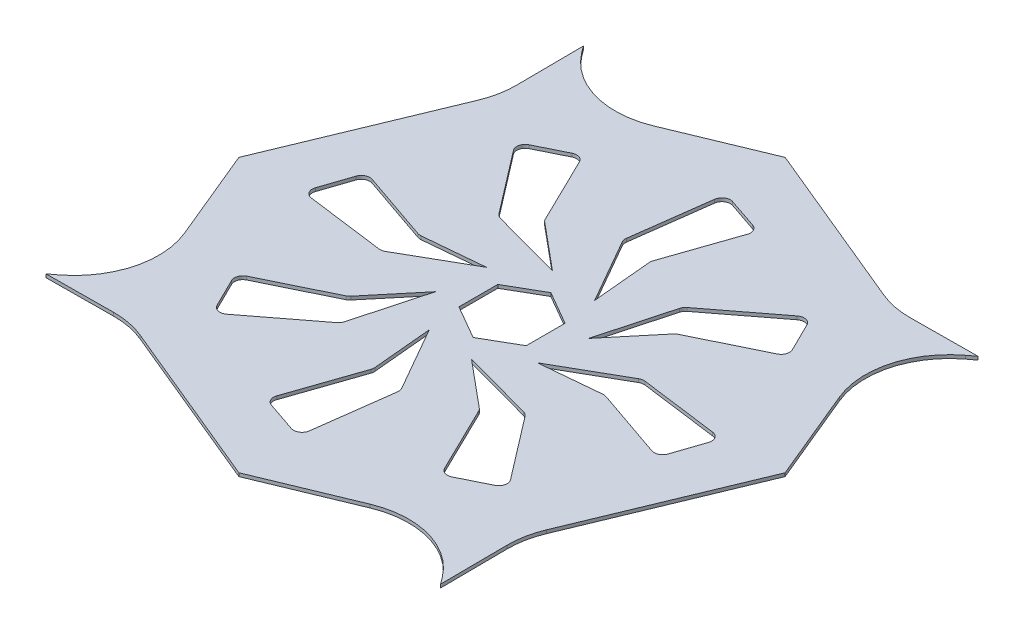
SolidWorks part; units mm, degrees
material "45"
ref_plane "Front Plane" through (0, 0, 0) normal (0, 0, 1) x (1, 0, 0)
ref_plane "Top Plane" through (0, 0, 0) normal (0, 1, 0) x (1, 0, 0)
ref_plane "Right Plane" through (0, 0, 0) normal (1, 0, 0) x (0, 0, -1)
sketch "Sketch1" plane through (0, 0, 0) normal (0, 1, 0) x (1, 0, 0)
  line L1 (114.805, -114.805) -> (162.3588, 0)
  line L2 (162.3588, 0) -> (114.805, 114.805)
  line L3 (114.805, 114.805) -> (0, 162.3588)
  line L4 (0, 162.3588) -> (-114.805, 114.805)
  line L5 (-114.805, 114.805) -> (-162.3588, 0)
  line L6 (-162.3588, 0) -> (-114.805, -114.805)
  line L7 (-114.805, -114.805) -> (0, -162.3588)
  line L8 (0, -162.3588) -> (114.805, -114.805)
  circle A0 centre (0, 0) radius 150 construction
  dimension "D1" = 300
extrude "Boss-Extrude1" add sketch "Sketch1" along normal blind 2
sketch "Sketch2" plane through (0, 2, 0) normal (0, 1, 0) x (1, 0, 0)
  line L0 (0, 0) -> (46.3685, 0) construction
  line L1 (20, 11.547) -> (0, 23.094)
  line L2 (0, 23.094) -> (-20, 11.547)
  line L3 (-20, 11.547) -> (-20, -11.547)
  line L4 (-20, -11.547) -> (0, -23.094)
  line L5 (0, -23.094) -> (20, -11.547)
  line L6 (20, -11.547) -> (20, 11.547)
  line L7 (0, 0) -> (20, -11.547) construction
  circle A0 centre (0, 0) radius 20 construction
  dimension "D1" = 40
  dimension "D2" = 30
extrude "Cut-Extrude1" cut sketch "Sketch2" against normal blind 10
sketch "Sketch3" plane through (0, 2, 0) normal (0, 1, 0) x (1, 0, 0)
  line L0 (7.1807, 123.975) -> (25.2073, 117.8588)
  line L1 (28.3287, 111.4971) -> (13.9987, 69.8505)
  line L2 (13.7476, 67.7664) -> (17.0204, 32.1308)
  line L3 (17.0204, 32.1308) -> (-4.8848, 70.4296)
  line L4 (-5.5015, 73.5667) -> (0.6173, 119.8948)
  line L5 (92.7411, 82.586) -> (101.163, 65.5145)
  line L6 (98.8718, 58.8089) -> (59.2903, 39.4932)
  line L7 (57.6391, 38.197) -> (34.7552, 10.6847)
  line L8 (34.7552, 10.6847) -> (46.3472, 53.2553)
  line L9 (48.1294, 55.9097) -> (85.2149, 84.3419)
  line L10 (123.975, -7.1807) -> (117.8588, -25.2073)
  line L11 (111.4971, -28.3287) -> (69.8505, -13.9987)
  line L12 (67.7664, -13.7476) -> (32.1308, -17.0204)
  line L13 (32.1308, -17.0204) -> (70.4296, 4.8848)
  line L14 (73.5667, 5.5015) -> (119.8948, -0.6173)
  line L15 (82.586, -92.7411) -> (65.5145, -101.163)
  line L16 (58.8089, -98.8718) -> (39.4932, -59.2903)
  line L17 (38.197, -57.6391) -> (10.6847, -34.7552)
  line L18 (10.6847, -34.7552) -> (53.2553, -46.3472)
  line L19 (55.9097, -48.1294) -> (84.3419, -85.2149)
  line L20 (-7.1807, -123.975) -> (-25.2073, -117.8588)
  line L21 (-28.3287, -111.4971) -> (-13.9987, -69.8505)
  line L22 (-13.7476, -67.7664) -> (-17.0204, -32.1308)
  line L23 (-17.0204, -32.1308) -> (4.8848, -70.4296)
  line L24 (5.5015, -73.5667) -> (-0.6173, -119.8948)
  line L25 (-92.7411, -82.586) -> (-101.163, -65.5145)
  line L26 (-98.8718, -58.8089) -> (-59.2903, -39.4932)
  line L27 (-57.6391, -38.197) -> (-34.7552, -10.6847)
  line L28 (-34.7552, -10.6847) -> (-46.3472, -53.2553)
  line L29 (-48.1294, -55.9097) -> (-85.2149, -84.3419)
  line L30 (-123.975, 7.1807) -> (-117.8588, 25.2073)
  line L31 (-111.4971, 28.3287) -> (-69.8505, 13.9987)
  line L32 (-67.7664, 13.7476) -> (-32.1308, 17.0204)
  line L33 (-32.1308, 17.0204) -> (-70.4296, -4.8848)
  line L34 (-73.5667, -5.5015) -> (-119.8948, 0.6173)
  line L35 (-82.586, 92.7411) -> (-65.5145, 101.163)
  line L36 (-58.8089, 98.8718) -> (-39.4932, 59.2903)
  line L37 (-38.197, 57.6391) -> (-10.6847, 34.7552)
  line L38 (-10.6847, 34.7552) -> (-53.2553, 46.3472)
  line L39 (-55.9097, 48.1294) -> (-84.3419, 85.2149)
  arc A0 (13.9987, 69.8505) -> (13.7476, 67.7664) centre (18.7267, 68.2237) ccw
  arc A1 (-4.8848, 70.4296) -> (-5.5015, 73.5667) centre (-0.5445, 72.912) cw
  arc A2 (0.6173, 119.8948) -> (7.1807, 123.975) centre (5.5743, 119.2401) cw
  arc A3 (28.3287, 111.4971) -> (25.2073, 117.8588) centre (23.6008, 113.1239) ccw
  circle A4 centre (0, 0) radius 14.7187 construction
  arc A5 (59.2903, 39.4932) -> (57.6391, 38.197) centre (61.4832, 34.9997) ccw
  arc A6 (46.3472, 53.2553) -> (48.1294, 55.9097) centre (51.1715, 51.9416) cw
  arc A7 (85.2149, 84.3419) -> (92.7411, 82.586) centre (88.2571, 80.3739) cw
  arc A8 (98.8718, 58.8089) -> (101.163, 65.5145) centre (96.679, 63.3024) ccw
  arc A9 (69.8505, -13.9987) -> (67.7664, -13.7476) centre (68.2237, -18.7267) ccw
  arc A10 (70.4296, 4.8848) -> (73.5667, 5.5015) centre (72.912, 0.5445) cw
  arc A11 (119.8948, -0.6173) -> (123.975, -7.1807) centre (119.2401, -5.5743) cw
  arc A12 (111.4971, -28.3287) -> (117.8588, -25.2073) centre (113.1239, -23.6008) ccw
  arc A13 (39.4932, -59.2903) -> (38.197, -57.6391) centre (34.9997, -61.4832) ccw
  arc A14 (53.2553, -46.3472) -> (55.9097, -48.1294) centre (51.9416, -51.1715) cw
  arc A15 (84.3419, -85.2149) -> (82.586, -92.7411) centre (80.3739, -88.2571) cw
  arc A16 (58.8089, -98.8718) -> (65.5145, -101.163) centre (63.3024, -96.679) ccw
  arc A17 (-13.9987, -69.8505) -> (-13.7476, -67.7664) centre (-18.7267, -68.2237) ccw
  arc A18 (4.8848, -70.4296) -> (5.5015, -73.5667) centre (0.5445, -72.912) cw
  arc A19 (-0.6173, -119.8948) -> (-7.1807, -123.975) centre (-5.5743, -119.2401) cw
  arc A20 (-28.3287, -111.4971) -> (-25.2073, -117.8588) centre (-23.6008, -113.1239) ccw
  arc A21 (-59.2903, -39.4932) -> (-57.6391, -38.197) centre (-61.4832, -34.9997) ccw
  arc A22 (-46.3472, -53.2553) -> (-48.1294, -55.9097) centre (-51.1715, -51.9416) cw
  arc A23 (-85.2149, -84.3419) -> (-92.7411, -82.586) centre (-88.2571, -80.3739) cw
  arc A24 (-98.8718, -58.8089) -> (-101.163, -65.5145) centre (-96.679, -63.3024) ccw
  arc A25 (-69.8505, 13.9987) -> (-67.7664, 13.7476) centre (-68.2237, 18.7267) ccw
  arc A26 (-70.4296, -4.8848) -> (-73.5667, -5.5015) centre (-72.912, -0.5445) cw
  arc A27 (-119.8948, 0.6173) -> (-123.975, 7.1807) centre (-119.2401, 5.5743) cw
  arc A28 (-111.4971, 28.3287) -> (-117.8588, 25.2073) centre (-113.1239, 23.6008) ccw
  arc A29 (-39.4932, 59.2903) -> (-38.197, 57.6391) centre (-34.9997, 61.4832) ccw
  arc A30 (-53.2553, 46.3472) -> (-55.9097, 48.1294) centre (-51.9416, 51.1715) cw
  arc A31 (-84.3419, 85.2149) -> (-82.586, 92.7411) centre (-80.3739, 88.2571) cw
  arc A32 (-58.8089, 98.8718) -> (-65.5145, 101.163) centre (-63.3024, 96.679) ccw
  point P110 (0, 0)
  dimension "D1" = 5
  dimension "D2" = 8
extrude "Cut-Extrude2" cut sketch "Sketch3" against normal blind 10
sketch "Sketch6" plane through (0, 2, 0) normal (0, 1, 0) x (1, 0, 0)
  line L0 (0, 0) -> (-114.805, 114.805) construction
  line L1 (-116.9103, 109.7225) -> (-117.2961, 159.7225)
  line L2 (-114.805, 114.805) -> (-162.3588, 0) construction
  line L3 (-117.2961, 159.7225) -> (-90.8359, 124.7334)
  line L4 (0, 162.3588) -> (-114.805, 114.805) construction
  line L5 (-90.8359, 124.7334) -> (-114.805, 114.805)
  line L6 (-114.805, 114.805) -> (-116.9103, 109.7225)
  line L7 (109.7225, 116.9103) -> (159.7225, 117.2961)
  line L8 (159.7225, 117.2961) -> (124.7334, 90.8359)
  line L9 (124.7334, 90.8359) -> (114.805, 114.805)
  line L10 (114.805, 114.805) -> (109.7225, 116.9103)
  line L11 (0, 0) -> (114.805, 114.805) construction
  line L12 (116.9103, -109.7225) -> (117.2961, -159.7225)
  line L13 (117.2961, -159.7225) -> (90.8359, -124.7334)
  line L14 (90.8359, -124.7334) -> (114.805, -114.805)
  line L15 (114.805, -114.805) -> (116.9103, -109.7225)
  line L16 (0, 0) -> (114.805, -114.805) construction
  line L17 (-109.7225, -116.9103) -> (-159.7225, -117.2961)
  line L18 (-159.7225, -117.2961) -> (-124.7334, -90.8359)
  line L19 (-124.7334, -90.8359) -> (-114.805, -114.805)
  line L20 (-114.805, -114.805) -> (-109.7225, -116.9103)
  line L21 (0, 0) -> (-114.805, -114.805) construction
  circle A0 centre (0, 0) radius 96.6837 construction
  point P27 (0, 0)
  dimension "D1" = 4
  dimension "D2" = 50
  dimension "D3" = 30
extrude "Boss-Extrude2" add sketch "Sketch6" against normal blind 2
fillet "Fillet1" radius 50 8 edges at (-116.9103, 1, -109.7225) (-90.8359, 1, -124.7334) (-124.7334, 1, 90.8359) (-109.7225, 1, 116.9103) (90.8359, 1, 124.7334) (116.9103, 1, 109.7225) (109.7225, 1, -116.9103) (124.7334, 1, -90.8359)
